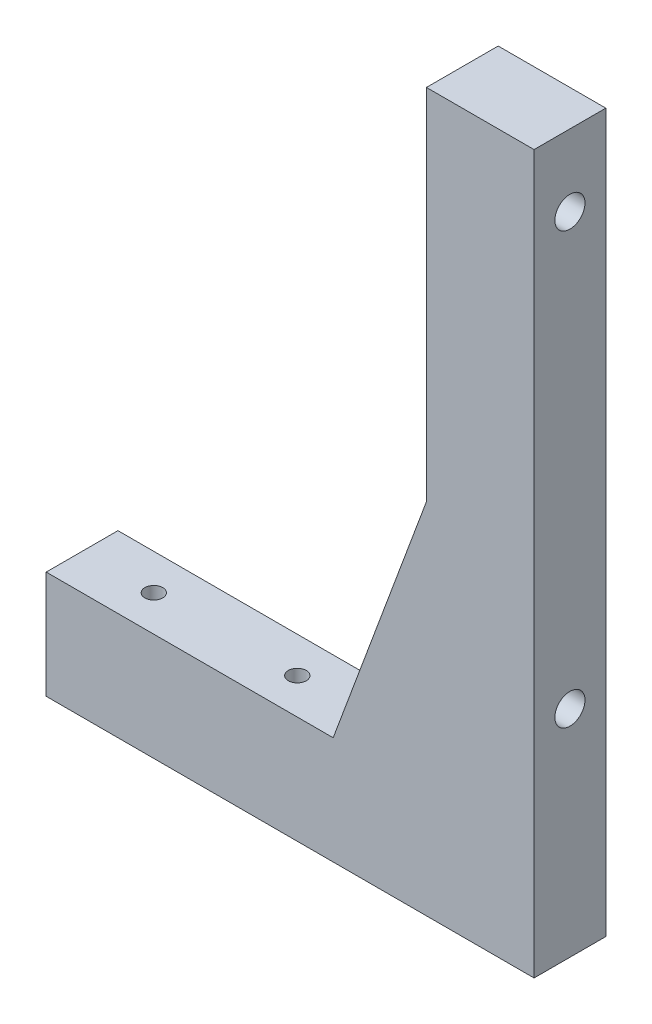
SolidWorks part; units mm, degrees
material "6061 合金"
ref_plane "前视基准面" through (0, 0, 0) normal (0, 0, 1) x (1, 0, 0)
ref_plane "上视基准面" through (0, 0, 0) normal (0, 1, 0) x (1, 0, 0)
ref_plane "右视基准面" through (0, 0, 0) normal (1, 0, 0) x (0, 0, -1)
sketch "草图1" plane through (0, 0, 0) normal (0, 0, 1) x (1, 0, 0)
  line L0 (-68, 0) -> (-68, 15)
  line L1 (-68, 15) -> (-28, 15)
  line L2 (-28, 15) -> (-15, 50)
  line L3 (-15, 50) -> (-15, 100)
  line L4 (-15, 100) -> (0, 100)
  line L5 (0, 100) -> (0, 0)
  line L6 (0, 0) -> (-68, 0)
  dimension "D1" = 68
  dimension "D2" = 100
  dimension "D3" = 15
  dimension "D4" = 15
  dimension "D5" = 40
  dimension "D6" = 50
extrude "凸台-拉伸1" add sketch "草图1" along normal mid plane 10
hole_wizard "M5 螺纹孔1" positions "草图7" profile "草图8" tap size "M5" standard "GB"
sketch "草图7" plane through (0, 0, 0) normal (0, -1, 0) x (-1, 0, 0)
  line L0 (68, -5) -> (68, 5) construction
  point P0 (49, 0)
  point P2 (19, 0)
  dimension "D1" = 30
  dimension "D2" = 19
sketch "草图8" plane through (-49, 0, 0) normal (1, 0, 0) x (0, 0, -1)
  line L0 (0, 0) -> (0, 14.2618)
  line L1 (0, 14.2618) -> (2.1, 13)
  line L2 (2.1, 13) -> (2.1, 0)
  line L5 (2.1, 0) -> (0, 0)
  line L10 (0, 14.2618) -> (-2.1, 13) construction
  line L11 (0, -6.35) -> (0, 107.95) construction
  dimension "螺纹孔钻头直径" = 4.2
  dimension "螺纹孔钻头深度" = 13
  dimension "导头角度" = 118
cosmetic thread "孔螺蚊线1" parameters "D1"=10, "D2"=5
cosmetic thread "孔螺蚊线2" parameters "D1"=10, "D2"=5
hole_wizard "M5 螺纹孔2" positions "草图10" profile "草图9" tap size "M5" standard "GB"
sketch "草图10" plane through (0, 0, 0) normal (1, 0, 0) x (0, 0, -1)
  line L0 (-5, 0) -> (5, 0) construction
  point P0 (0, 30)
  point P2 (0, 90)
  dimension "D1" = 60
  dimension "D2" = 30
sketch "草图9" plane through (0, 30, 0) normal (0, 1, 0) x (0, 0, -1)
  line L0 (0, 0) -> (0, 15.2618)
  line L1 (0, 15.2618) -> (2.1, 14)
  line L2 (2.1, 14) -> (2.1, 0)
  line L5 (2.1, 0) -> (0, 0)
  line L10 (0, 15.2618) -> (-2.1, 14) construction
  line L11 (0, -6.35) -> (0, 107.95) construction
  dimension "螺纹孔钻头直径" = 4.2
  dimension "螺纹孔钻头深度" = 14
  dimension "导头角度" = 118
cosmetic thread "孔螺蚊线3" parameters "D1"=10, "D2"=5
cosmetic thread "孔螺蚊线4" parameters "D1"=10, "D2"=5
hole_wizard "M3 螺纹孔1" positions "草图12" profile "草图11" tap size "M3" standard "GB"
sketch "草图12" plane through (0, 15, 0) normal (0, 1, 0) x (1, 0, 0)
  line L0 (-68, -5) -> (-68, 5) construction
  line L1 (-28, 5) -> (-68, 5) construction
  point P0 (-58, 0)
  point P2 (-38, 0)
  dimension "D1" = 10
  dimension "D2" = 20
  dimension "D3" = 5
sketch "草图11" plane through (-58, 15, 0) normal (1, 0, 0) x (0, 0, 1)
  line L0 (0, 0) -> (0, 13.2511)
  line L1 (0, 13.2511) -> (1.25, 12.5)
  line L2 (1.25, 12.5) -> (1.25, 0)
  line L5 (1.25, 0) -> (0, 0)
  line L10 (0, 13.2511) -> (-1.25, 12.5) construction
  line L11 (0, -6.35) -> (0, 107.95) construction
  dimension "螺纹孔钻头直径" = 2.5
  dimension "螺纹孔钻头深度" = 12.5
  dimension "导头角度" = 118
cosmetic thread "孔螺蚊线5" parameters "D1"=10, "D2"=3
cosmetic thread "孔螺蚊线6" parameters "D1"=10, "D2"=3
